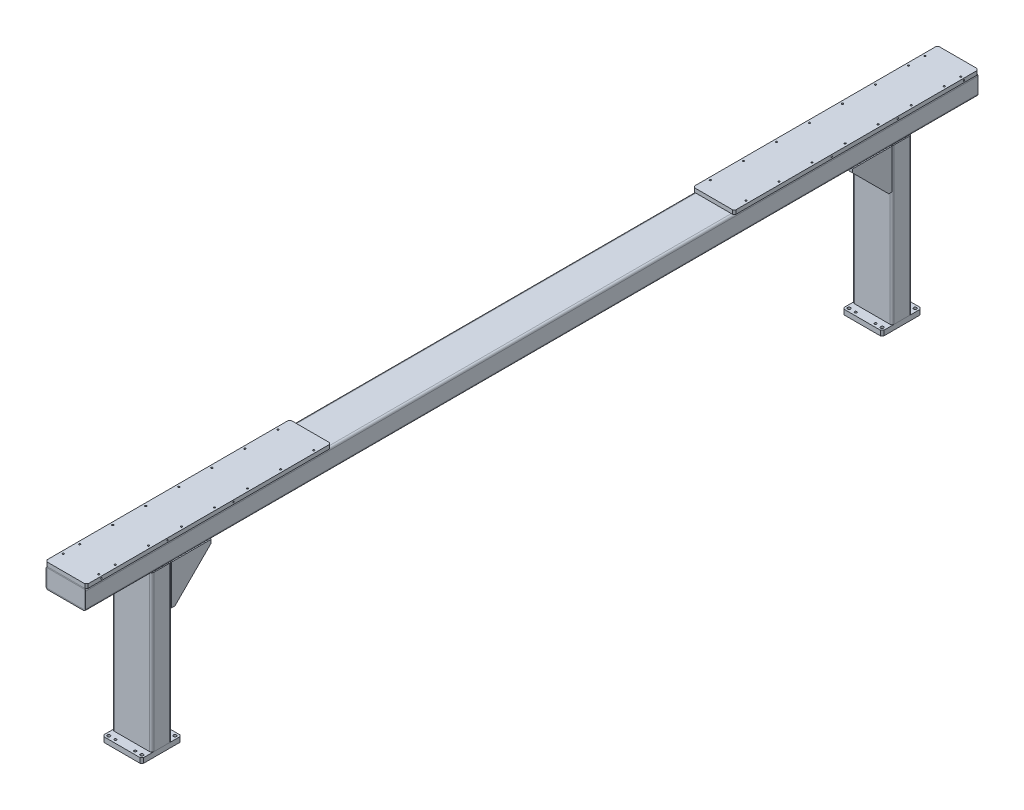
SolidWorks part; units mm, degrees
material "Q235A"
ref_plane "前基準面" through (0, 0, 0) normal (0, 0, 1) x (1, 0, 0)
ref_plane "上基準面" through (0, 0, 0) normal (0, 1, 0) x (1, 0, 0)
ref_plane "右基準面" through (0, 0, 0) normal (1, 0, 0) x (0, 0, -1)
sketch "草图1" plane through (0, 0, 0) normal (1, 0, 0) x (0, 0, -1)
  line L0 (0, 500) -> (0, 0) construction
  line L1 (-1350, 500) -> (1350, 500)
  line L2 (-1120, 500) -> (-1120, 0)
  line L4 (1120, 500) -> (1120, 0)
  line L5 (-1350, 500) -> (1350, 500)
  dimension "D1" = 500
  dimension "D2" = 2700
  dimension "D3" = 230
other "矩型管 120 X 60 X 3.2(1)"
ref_plane "基准面1" through (0, 500, -1120) normal (0, -1, 0) x (0, 0, -1)
sketch "Sketch12" plane through (0, 500, -1120) normal (0, -1, 0) x (0, 0, -1)
  line L0 (-23.6, -56.8) -> (23.6, -56.8)
  line L1 (-26.8, -53.6) -> (-26.8, 53.6)
  line L2 (23.6, 56.8) -> (-23.6, 56.8)
  line L3 (26.8, 53.6) -> (26.8, -53.6)
  line L4 (-23.6, -60) -> (23.6, -60)
  line L5 (-30, -53.6) -> (-30, 53.6)
  line L6 (23.6, 60) -> (-23.6, 60)
  line L7 (30, 53.6) -> (30, -53.6)
  line L8 (-30, 0) -> (-26.8, 0) construction
  line L9 (-26.8, 0) -> (26.8, 0) construction
  line L10 (26.8, 0) -> (30, 0) construction
  line L11 (0, 60) -> (0, 56.8) construction
  line L12 (0, 56.8) -> (0, -56.8) construction
  line L13 (0, -56.8) -> (0, -60) construction
  arc A0 (30, 53.6) -> (23.6, 60) centre (23.6, 53.6) ccw
  arc A1 (23.6, -60) -> (30, -53.6) centre (23.6, -53.6) ccw
  arc A2 (-30, -53.6) -> (-23.6, -60) centre (-23.6, -53.6) ccw
  arc A3 (-23.6, 60) -> (-30, 53.6) centre (-23.6, 53.6) ccw
  arc A4 (-23.6, 56.8) -> (-26.8, 53.6) centre (-23.6, 53.6) ccw
  arc A5 (26.8, 53.6) -> (23.6, 56.8) centre (23.6, 53.6) ccw
  arc A6 (23.6, -56.8) -> (26.8, -53.6) centre (23.6, -53.6) ccw
  arc A7 (-26.8, -53.6) -> (-23.6, -56.8) centre (-23.6, -53.6) ccw
  point P6 (-30, 60)
  point P33 (-30, -60)
  point P34 (30, -60)
  point P36 (30, 60)
  point P37 (0, 0)
  dimension "D1" = 6.4
  dimension "Thickness" = 3.2
  dimension "V_leg" = 120
  dimension "H_leg" = 60
other "矩型管 120 X 60 X 3.2(2)"
ref_plane "基准面2" through (0, 500, 1350) normal (0, 0, -1) x (0, 1, 0)
sketch "Sketch1" plane through (0, 500, 1350) normal (0, 0, -1) x (0, 1, 0)
  line L0 (-23.6, -56.8) -> (23.6, -56.8)
  line L1 (-26.8, -53.6) -> (-26.8, 53.6)
  line L2 (23.6, 56.8) -> (-23.6, 56.8)
  line L3 (26.8, 53.6) -> (26.8, -53.6)
  line L4 (-23.6, -60) -> (23.6, -60)
  line L5 (-30, -53.6) -> (-30, 53.6)
  line L6 (23.6, 60) -> (-23.6, 60)
  line L7 (30, 53.6) -> (30, -53.6)
  line L8 (-30, 0) -> (-26.8, 0) construction
  line L9 (-26.8, 0) -> (26.8, 0) construction
  line L10 (26.8, 0) -> (30, 0) construction
  line L11 (0, 60) -> (0, 56.8) construction
  line L12 (0, 56.8) -> (0, -56.8) construction
  line L13 (0, -56.8) -> (0, -60) construction
  arc A0 (30, 53.6) -> (23.6, 60) centre (23.6, 53.6) ccw
  arc A1 (23.6, -60) -> (30, -53.6) centre (23.6, -53.6) ccw
  arc A2 (-30, -53.6) -> (-23.6, -60) centre (-23.6, -53.6) ccw
  arc A3 (-23.6, 60) -> (-30, 53.6) centre (-23.6, 53.6) ccw
  arc A4 (-23.6, 56.8) -> (-26.8, 53.6) centre (-23.6, 53.6) ccw
  arc A5 (26.8, 53.6) -> (23.6, 56.8) centre (23.6, 53.6) ccw
  arc A6 (23.6, -56.8) -> (26.8, -53.6) centre (23.6, -53.6) ccw
  arc A7 (-26.8, -53.6) -> (-23.6, -56.8) centre (-23.6, -53.6) ccw
  point P6 (-30, 60)
  point P33 (-30, -60)
  point P34 (30, -60)
  point P36 (30, 60)
  point P37 (0, 0)
  dimension "D1" = 6.4
  dimension "Thickness" = 3.2
  dimension "V_leg" = 120
  dimension "H_leg" = 60
other "剪裁/延伸1"
sketch "草图4" plane through (0, 530, 0) normal (0, 1, 0) x (1, 0, 0)
  line L5 (0, 0) -> (0, 550.3028) construction
  line L31 (-62.5, 610) -> (-62.5, 1350)
  line L32 (-62.5, 610) -> (62.5, 610)
  line L34 (62.5, 610) -> (62.5, 1350)
  line L35 (-62.5, 1350) -> (62.5, 1350)
  line L45 (-53.6, 1350) -> (53.6, 1350) construction
  dimension "D1" = 125
  dimension "D3" = 740
extrude "凸台-拉伸1" add sketch "草图4" along normal blind 12 separate body
sketch "草图5" plane through (0, 0, 0) normal (0, -1, 0) x (1, 0, 0)
  line L0 (0, 0) -> (0, 592.2085) construction
  line L1 (-60, 1180) -> (60, 1180)
  line L2 (-60, 1180) -> (-60, 1060)
  line L3 (-60, 1060) -> (60, 1060)
  line L4 (60, 1180) -> (60, 1060)
  line L5 (0, 0) -> (-186.7981, 0) construction
  line L7 (-60, 1120) -> (60, 1120) construction
  line L12 (60, -1180) -> (60, -1060)
  line L13 (-60, 1143.6) -> (-60, 1096.4) construction
  line L14 (60, 1096.4) -> (60, 1143.6) construction
  line L19 (-60, -1060) -> (60, -1060)
  line L20 (-60, -1180) -> (-60, -1060)
  line L21 (-60, -1180) -> (60, -1180)
  dimension "D1" = 120
extrude "凸台-拉伸2" add sketch "草图5" along normal blind 15 separate body
hole_wizard "Ø9.0 (9) 直径孔1" positions "草图14" profile "草图15" hole size "Ø9.0" standard "GB"
sketch "草图14" plane through (0, -15, 0) normal (0, 1, 0) x (1, 0, 0)
  line L0 (-60, 1120) -> (-147.8324, 1120) construction
  line L4 (0, 0) -> (-119.1447, 0) construction
  line L8 (0, 0) -> (0, 84.4415) construction
  line L9 (-60, 1060) -> (-60, 1180) construction
  point P0 (-50, 1170)
  point P22 (-50, 1070)
  point P23 (50, 1070)
  point P24 (50, 1170)
  point P25 (50, -1170)
  point P26 (50, -1070)
  point P27 (-50, -1070)
  point P28 (-50, -1170)
  dimension "D1" = 100
  dimension "D2" = 100
sketch "草图15" plane through (-50, -15, -1170) normal (1, 0, 0) x (0, 0, -1)
  line L0 (0, 0) -> (0, 22.7039)
  line L1 (0, 22.7039) -> (4.5, 20)
  line L2 (4.5, 20) -> (4.5, 0)
  line L5 (4.5, 0) -> (0, 0)
  line L10 (0, 22.7039) -> (-4.5, 20) construction
  line L11 (0, -6.35) -> (0, 107.95) construction
  dimension "孔直径" = 9
  dimension "孔深度" = 20
  dimension "导头角度" = 118
hole_wizard "M8 螺纹孔1" positions "草图12" profile "草图13" tap size "M8" standard "GB"
sketch "草图12" plane through (0, 0, 0) normal (0, 1, 0) x (1, 0, 0)
  line L1 (-60, 1120) -> (-136.759, 1120) construction
  line L5 (0, 0) -> (0, 90.6038) construction
  line L8 (0, 0) -> (-112.8839, 0) construction
  line L9 (-60, 1060) -> (-60, 1180) construction
  point P0 (-30, 1070)
  point P21 (-30, 1170)
  point P22 (30, 1170)
  point P23 (30, 1070)
  point P24 (30, -1070)
  point P25 (30, -1170)
  point P26 (-30, -1170)
  point P27 (-30, -1070)
  dimension "40" = 100
  dimension "D2" = 60
cosmetic thread "孔螺蚊线126"
cosmetic thread "孔螺蚊线127"
cosmetic thread "孔螺蚊线128"
cosmetic thread "孔螺蚊线129"
cosmetic thread "孔螺蚊线130"
cosmetic thread "孔螺蚊线131"
cosmetic thread "孔螺蚊线132"
cosmetic thread "孔螺蚊线133"
sketch "草图13" plane through (-30, 0, -1070) normal (1, 0, 0) x (0, 0, 1)
  line L0 (0, 0) -> (0, 24.2929)
  line L1 (0, 24.2929) -> (3.4, 22.25)
  line L2 (3.4, 22.25) -> (3.4, 0)
  line L5 (3.4, 0) -> (0, 0)
  line L10 (0, 24.2929) -> (-3.4, 22.25) construction
  line L11 (0, -6.35) -> (0, 107.95) construction
  dimension "螺纹孔钻头直径" = 6.8
  dimension "螺纹孔钻头深度" = 22.25
  dimension "导头角度" = 118
chamfer "倒角1" distance 5 angle 45 4 edges at (-60, -7.5, 1060) (-60, -7.5, 1180) (60, -7.5, 1060) (60, -7.5, 1180)
hole_wizard "M6 螺纹孔1" positions "草图24" profile "草图25" tap size "M6" standard "GB"
sketch "草图24" plane through (0, 542, 0) normal (0, 1, 0) x (1, 0, 0)
  line L0 (0, 610) -> (0, 80.7594) construction
  line L1 (-62.5, 610) -> (62.5, 610) construction
  point P0 (54, 654)
  point P8 (-54, 654)
  point P9 (-54, 754)
  point P10 (-54, 854)
  point P11 (-54, 954)
  point P12 (-54, 1054)
  point P13 (-54, 1154)
  point P14 (54, 754)
  point P15 (54, 854)
  point P16 (54, 954)
  point P17 (54, 1054)
  point P18 (54, 1154)
  point P27 (54, 1304)
  point P30 (-54, 1304)
  point P31 (54, 1254)
  point P32 (-54, 1254)
  dimension "D1" = 2
  dimension "D3" = 108
  dimension "D4" = 44
  dimension "D5" = 100
  dimension "D6" = 50
  dimension "D2" = 7
sketch "草图25" plane through (54, 542, -654) normal (1, 0, 0) x (0, 0, 1)
  line L0 (0, 0) -> (0, 16.5022)
  line L1 (0, 16.5022) -> (2.5, 15)
  line L2 (2.5, 15) -> (2.5, 0)
  line L5 (2.5, 0) -> (0, 0)
  line L10 (0, 16.5022) -> (-2.5, 15) construction
  line L11 (0, -6.35) -> (0, 107.95) construction
  dimension "螺纹孔钻头直径" = 5
  dimension "螺纹孔钻头深度" = 15
  dimension "导头角度" = 118
cosmetic thread "孔螺蚊线47"
cosmetic thread "孔螺蚊线48"
cosmetic thread "孔螺蚊线49"
cosmetic thread "孔螺蚊线50"
cosmetic thread "孔螺蚊线51"
cosmetic thread "孔螺蚊线52"
cosmetic thread "孔螺蚊线53"
cosmetic thread "孔螺蚊线54"
cosmetic thread "孔螺蚊线55"
cosmetic thread "孔螺蚊线56"
cosmetic thread "孔螺蚊线57"
cosmetic thread "孔螺蚊线58"
cosmetic thread "孔螺蚊线59"
cosmetic thread "孔螺蚊线60"
cosmetic thread "孔螺蚊线64"
cosmetic thread "孔螺蚊线65"
chamfer "倒角3" distance 5 angle 45 4 edges at (-62.5, 536, -1350) (62.5, 536, -1350) (-62.5, 536, -610) (62.5, 536, -610)
hole_wizard "M5 螺纹孔1" positions "草图26" profile "草图27" tap size "M5" standard "GB"
sketch "草图26" plane through (62.5, 0, 0) normal (1, 0, 0) x (0, 0, -1)
  line L0 (610, 530) -> (610, 542) construction
  line L1 (615, 542) -> (1345, 542) construction
  point P0 (905, 536)
  point P4 (1105, 536)
  point P5 (1305, 536)
  dimension "D2" = 295
  dimension "D3" = 200
  dimension "D4" = 6
  dimension "D1" = 3
sketch "草图27" plane through (62.5, 536, -905) normal (0, 1, 0) x (0, 0, -1)
  line L0 (0, 0) -> (0, 13.6618)
  line L1 (0, 13.6618) -> (2.1, 12.4)
  line L2 (2.1, 12.4) -> (2.1, 0)
  line L5 (2.1, 0) -> (0, 0)
  line L10 (0, 13.6618) -> (-2.1, 12.4) construction
  line L11 (0, -6.35) -> (0, 107.95) construction
  dimension "螺纹孔钻头直径" = 4.2
  dimension "螺纹孔钻头深度" = 12.4
  dimension "导头角度" = 118
cosmetic thread "孔螺蚊线61"
cosmetic thread "孔螺蚊线62"
cosmetic thread "孔螺蚊线63"
mirror "镜向1" about plane through (0, 0, 0) normal (1, 0, 0) of "M5 螺纹孔1"
ref_plane "基准面3" through (0, 0, -980) normal (0, 0, -1) x (-1, 0, 0)
mirror "镜向3" about plane through (0, 0, 0) normal (0, 0, 1) of bodies 154 156 155 157
chamfer "倒角4" distance 5 angle 45 4 edges at (-60, -7.5, -1180) (60, -7.5, -1180) (-60, -7.5, -1060) (60, -7.5, -1060)
sketch "草图32" plane through (-60, 0, 0) normal (-1, 0, 0) x (0, 0, 1)
  line L1 (-1330, 497) -> (-630, 497)
  line L2 (-1330, 497) -> (-1330, 482)
  line L3 (-1330, 482) -> (-630, 482)
  line L4 (-630, 497) -> (-630, 482)
  line L7 (0, 0) -> (0, 842.9899) construction
  line L8 (630, 497) -> (630, 482)
  line L9 (1330, 482) -> (630, 482)
  line L10 (1330, 497) -> (1330, 482)
  line L11 (1330, 497) -> (630, 497)
  line L12 (-1350, 530) -> (-1350, 542) construction
  line L13 (-1350, 470) -> (1350, 470) construction
  dimension "D1" = 15
  dimension "D2" = 20
  dimension "D3" = 700
  dimension "D4" = 12
extrude "凸台-拉伸3" add sketch "草图32" along normal blind 7 separate body
sketch "草图33" plane through (-67, 0, 0) normal (-1, 0, 0) x (0, 0, 1)
  line L0 (1330, 482) -> (1330, 497) construction
  line L1 (-1330, 497) -> (1330, 497)
  line L2 (-1330, 497) -> (-1330, 487)
  line L3 (-1330, 487) -> (1330, 487)
  line L4 (1330, 497) -> (1330, 487)
  line L5 (630, 482) -> (1330, 482) construction
  dimension "D1" = 5
extrude "切除-拉伸1" [suppressed] cut sketch "草图33" against normal blind 3
hole_wizard "M4 螺纹孔3" positions "草图34" profile "草图35" tap size "M4" standard "GB"
sketch "草图34" plane through (-67, 0, 0) normal (-1, 0, 0) x (0, 0, 1)
  line L3 (0, 874.3594) -> (0, 0) construction
  line L4 (-1330, 497) -> (-1330, 482) construction
  line L5 (-630, 497) -> (-1330, 497) construction
  point P0 (-1310, 489.5)
  point P6 (-1250, 489.5)
  point P7 (-1190, 489.5)
  point P8 (-1130, 489.5)
  point P9 (-1070, 489.5)
  point P10 (-1010, 489.5)
  point P11 (-950, 489.5)
  point P12 (-890, 489.5)
  point P13 (-830, 489.5)
  point P14 (-770, 489.5)
  point P15 (-710, 489.5)
  point P16 (-650, 489.5)
  point P27 (650, 489.5)
  point P28 (710, 489.5)
  point P29 (770, 489.5)
  point P30 (830, 489.5)
  point P31 (890, 489.5)
  point P32 (950, 489.5)
  point P33 (1010, 489.5)
  point P34 (1070, 489.5)
  point P35 (1130, 489.5)
  point P36 (1190, 489.5)
  point P37 (1250, 489.5)
  point P38 (1310, 489.5)
  dimension "D2" = 20
  dimension "D3" = 60
  dimension "D4" = 7.5
  dimension "D1" = 12
sketch "草图35" plane through (-67, 489.5, -1310) normal (0, 1, 0) x (0, 0, 1)
  line L0 (0, 0) -> (0, 11.0914)
  line L1 (0, 11.0914) -> (1.65, 10.1)
  line L2 (1.65, 10.1) -> (1.65, 0)
  line L5 (1.65, 0) -> (0, 0)
  line L10 (0, 11.0914) -> (-1.65, 10.1) construction
  line L11 (0, -6.35) -> (0, 107.95) construction
  dimension "螺纹孔钻头直径" = 3.3
  dimension "螺纹孔钻头深度" = 10.1
  dimension "导头角度" = 118
cosmetic thread "孔螺蚊线134"
cosmetic thread "孔螺蚊线135"
cosmetic thread "孔螺蚊线136"
cosmetic thread "孔螺蚊线137"
cosmetic thread "孔螺蚊线138"
cosmetic thread "孔螺蚊线139"
cosmetic thread "孔螺蚊线140"
cosmetic thread "孔螺蚊线141"
cosmetic thread "孔螺蚊线142"
cosmetic thread "孔螺蚊线143"
cosmetic thread "孔螺蚊线144"
cosmetic thread "孔螺蚊线145"
cosmetic thread "孔螺蚊线146"
cosmetic thread "孔螺蚊线147"
cosmetic thread "孔螺蚊线148"
cosmetic thread "孔螺蚊线149"
cosmetic thread "孔螺蚊线150"
cosmetic thread "孔螺蚊线151"
cosmetic thread "孔螺蚊线152"
cosmetic thread "孔螺蚊线153"
cosmetic thread "孔螺蚊线154"
cosmetic thread "孔螺蚊线155"
cosmetic thread "孔螺蚊线156"
cosmetic thread "孔螺蚊线157"
hole_wizard "M4 螺纹孔4" positions "草图36" profile "草图38" tap size "M4" standard "GB"
sketch "草图36" plane through (-67, 0, 0) normal (-1, 0, 0) x (0, 0, 1)
  line L3 (0, 0) -> (0, 707.483) construction
  line L8 (-980, 497) -> (-980, 521.2299) construction
  line L9 (-630, 497) -> (-1330, 497) construction
  line L11 (-1310, 489.5) -> (-1340, 489.5) construction
  line L13 (-1330, 497) -> (-1330, 482) construction
  point P0 (-1325, 489.5)
  point P8 (-635, 489.5)
  point P13 (635, 489.5)
  point P14 (1325, 489.5)
  dimension "D1" = 5
sketch "草图38" plane through (-67, 489.5, -1325) normal (0, 1, 0) x (0, 0, 1)
  line L0 (0, 0) -> (0, 11.0914)
  line L1 (0, 11.0914) -> (1.65, 10.1)
  line L2 (1.65, 10.1) -> (1.65, 0)
  line L5 (1.65, 0) -> (0, 0)
  line L10 (0, 11.0914) -> (-1.65, 10.1) construction
  line L11 (0, -6.35) -> (0, 107.95) construction
  dimension "螺纹孔钻头直径" = 3.3
  dimension "螺纹孔钻头深度" = 10.1
  dimension "导头角度" = 118
cosmetic thread "孔螺蚊线122"
cosmetic thread "孔螺蚊线123"
cosmetic thread "孔螺蚊线124"
cosmetic thread "孔螺蚊线125"
sketch "草图39" plane through (0, 0, -1350) normal (0, 0, -1) x (-1, 0, 0)
  line L0 (56.8, 476.4) -> (56.8, 523.6) construction
  line L1 (53.6, 526.8) -> (-53.6, 526.8) construction
  line L2 (-56.8, 523.6) -> (-56.8, 476.4) construction
  line L3 (-53.6, 473.2) -> (53.6, 473.2) construction
  line L4 (56.8, 476.4) -> (56.8, 523.6)
  line L5 (53.6, 526.8) -> (-53.6, 526.8)
  line L6 (-56.8, 523.6) -> (-56.8, 476.4)
  line L7 (-53.6, 473.2) -> (53.6, 473.2)
  arc A0 (56.8, 523.6) -> (53.6, 526.8) centre (53.6, 523.6) ccw construction
  arc A1 (-53.6, 526.8) -> (-56.8, 523.6) centre (-53.6, 523.6) ccw construction
  arc A2 (-56.8, 476.4) -> (-53.6, 473.2) centre (-53.6, 476.4) ccw construction
  arc A3 (53.6, 473.2) -> (56.8, 476.4) centre (53.6, 476.4) ccw construction
  arc A4 (56.8, 523.6) -> (53.6, 526.8) centre (53.6, 523.6) ccw
  arc A5 (-53.6, 526.8) -> (-56.8, 523.6) centre (-53.6, 523.6) ccw
  arc A6 (-56.8, 476.4) -> (-53.6, 473.2) centre (-53.6, 476.4) ccw
  arc A7 (53.6, 473.2) -> (56.8, 476.4) centre (53.6, 476.4) ccw
extrude "凸台-拉伸4" add sketch "草图39" against normal blind 5 separate body
mirror "镜向4" about plane through (0, 0, 0) normal (0, 0, 1) of bodies 184
sketch "草图40" plane through (60, 0, 0) normal (1, 0, 0) x (0, 0, -1)
  line L0 (-970, 470) -> (-1090, 470)
  line L1 (1350, 470) -> (-1350, 470) construction
  line L2 (-1090, 470) -> (-1090, 350)
  line L3 (-1090, 0) -> (-1090, 470) construction
  line L4 (-1090, 350) -> (-1080, 350)
  line L5 (-1080, 350) -> (-970, 460)
  line L6 (-970, 460) -> (-970, 470)
  dimension "D1" = 120
  dimension "D2" = 10
extrude "凸台-拉伸5" add sketch "草图40" against normal blind 10 separate body
mirror "镜向5" about plane through (0, 0, 0) normal (0, 0, 1) of bodies 186
